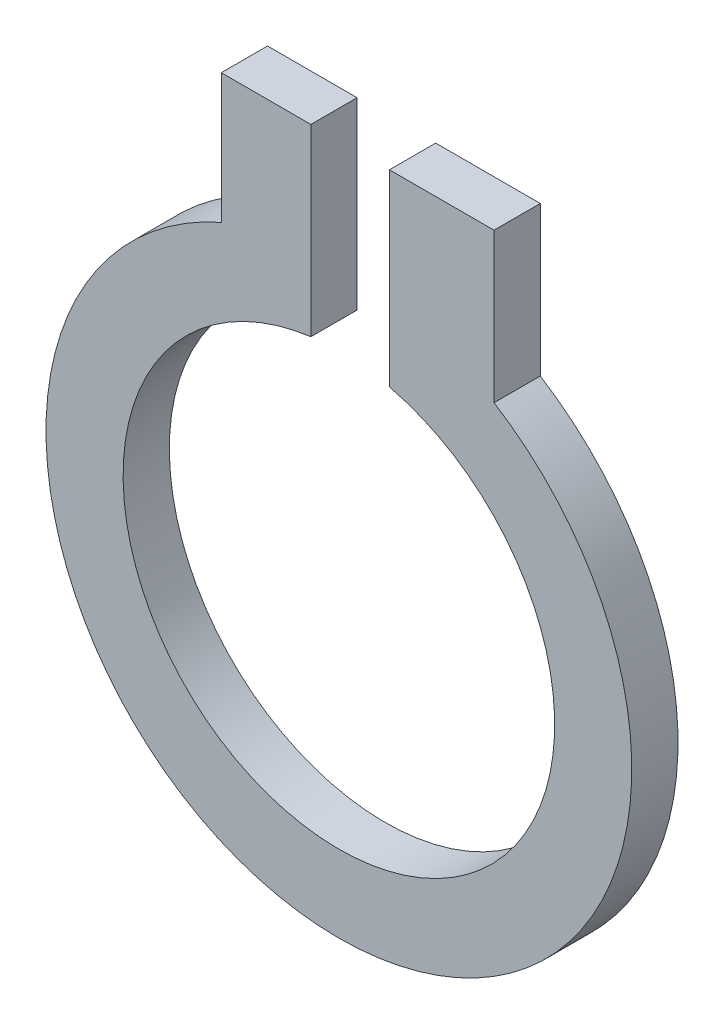
SolidWorks part; units mm, degrees
ref_plane "Front Plane" through (0, 0, 0) normal (0, 0, 1) x (1, 0, 0)
ref_plane "Top Plane" through (0, 0, 0) normal (0, 1, 0) x (1, 0, 0)
ref_plane "Right Plane" through (0, 0, 0) normal (1, 0, 0) x (0, 0, -1)
sketch "Sketch1" plane through (0, 0, 0) normal (0, 0, 1) x (1, 0, 0)
  line L0 (0.6559, 2.7221) -> (0.6559, 5.162)
  line L1 (0.6559, 5.162) -> (2.0129, 5.162)
  line L2 (2.0129, 5.162) -> (2.0129, 3.2231)
  line L3 (-0.3636, 2.7763) -> (-0.3636, 5.162)
  line L4 (-0.3636, 5.162) -> (-1.5259, 5.162)
  line L5 (-1.5259, 5.162) -> (-1.5259, 3.4802)
  arc A0 (-1.5259, 3.4802) -> (2.0129, 3.2231) centre (0, 0) ccw
  arc A1 (-0.3636, 2.7763) -> (0.6559, 2.7221) centre (0, 0) ccw
  dimension "D1" = 7.6
  dimension "D2" = 5.6
extrude "Boss-Extrude1" add sketch "Sketch1" along normal blind 0.6
